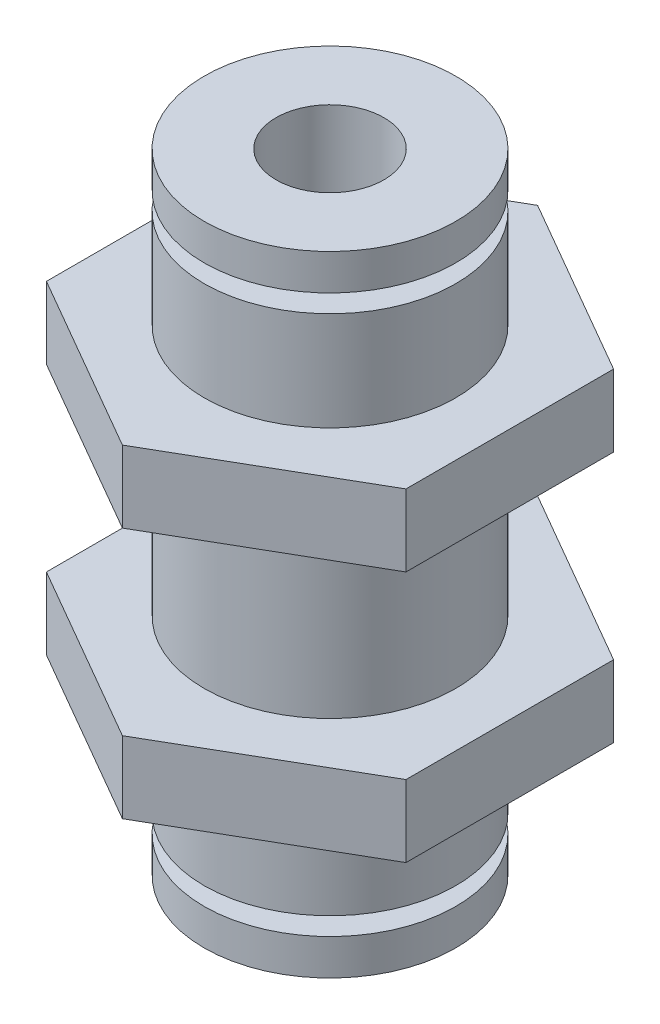
from build123d import *

# Parameters (mm, degrees)
SKETCH2_R           = 3
CUT_EXTRUDE1_DEPTH  = 37.373066959
SKETCH3_R           = 7
BOSS_EXTRUDE1_DEPTH = 4
BOSS_EXTRUDE2_START = -4
SKETCH4_R           = 7
BOSS_EXTRUDE2_DEPTH = 4


with BuildPart() as part:
    # Sketch1 → Revolve1 (revolve)
    with BuildSketch(Plane.XY, mode=Mode.PRIVATE) as revolve1_sk:
        Polygon((0, 17.5), (-7, 17.5), (-7, 15.5), (-5.5, 15.5), (-5.5, 14.5), (-7, 14.5), (-7, -14.5), (-5.5, -14.5), (-5.5, -15.5), (-7, -15.5), (-7, -17.5), (0, -17.5), align=None)
    revolve(revolve1_sk.sketch.rotate(Axis((0, 17.5, 0), (0, -1, 0)), 270), axis=Axis((0, 17.5, 0), (0, -1, 0)))

    # Sketch2 → Cut-Extrude1 (cut, through all)
    with BuildSketch(Plane(origin=(0, 17.5, 0), x_dir=(1, 0, 0), z_dir=(0, 1, 0))):
        with Locations(Location((0, 0, 0), (0, 0, 270))):
            Circle(SKETCH2_R)
    extrude(amount=-CUT_EXTRUDE1_DEPTH, mode=Mode.SUBTRACT)

    # Sketch4 → Boss-Extrude2 (add)
    with BuildSketch(Plane(origin=(0, -5, 0), x_dir=(1, 0, 0), z_dir=(0, 1, 0)).offset(BOSS_EXTRUDE2_START)):
        Polygon((0, 11.547005384), (-10, 5.773502692), (-10, -5.773502692), (0, -11.547005384), (10, -5.773502692), (10, 5.773502692), align=None)
        with Locations(Location((0, 0, 0), (0, 0, 270))):
            Circle(SKETCH4_R, mode=Mode.SUBTRACT)
    extrude(amount=BOSS_EXTRUDE2_DEPTH)


with BuildPart() as body_2:
    # Sketch3 → Boss-Extrude1 (new body)
    with BuildSketch(Plane(origin=(0, 5, 0), x_dir=(1, 0, 0), z_dir=(0, 1, 0))):
        Polygon((0, 11.547005384), (-10, 5.773502692), (-10, -5.773502692), (0, -11.547005384), (10, -5.773502692), (10, 5.773502692), align=None)
        with Locations(Location((0, 0, 0), (0, 0, 270))):
            Circle(SKETCH3_R, mode=Mode.SUBTRACT)
    extrude(amount=BOSS_EXTRUDE1_DEPTH)


solid = Compound([part.part, body_2.part])
